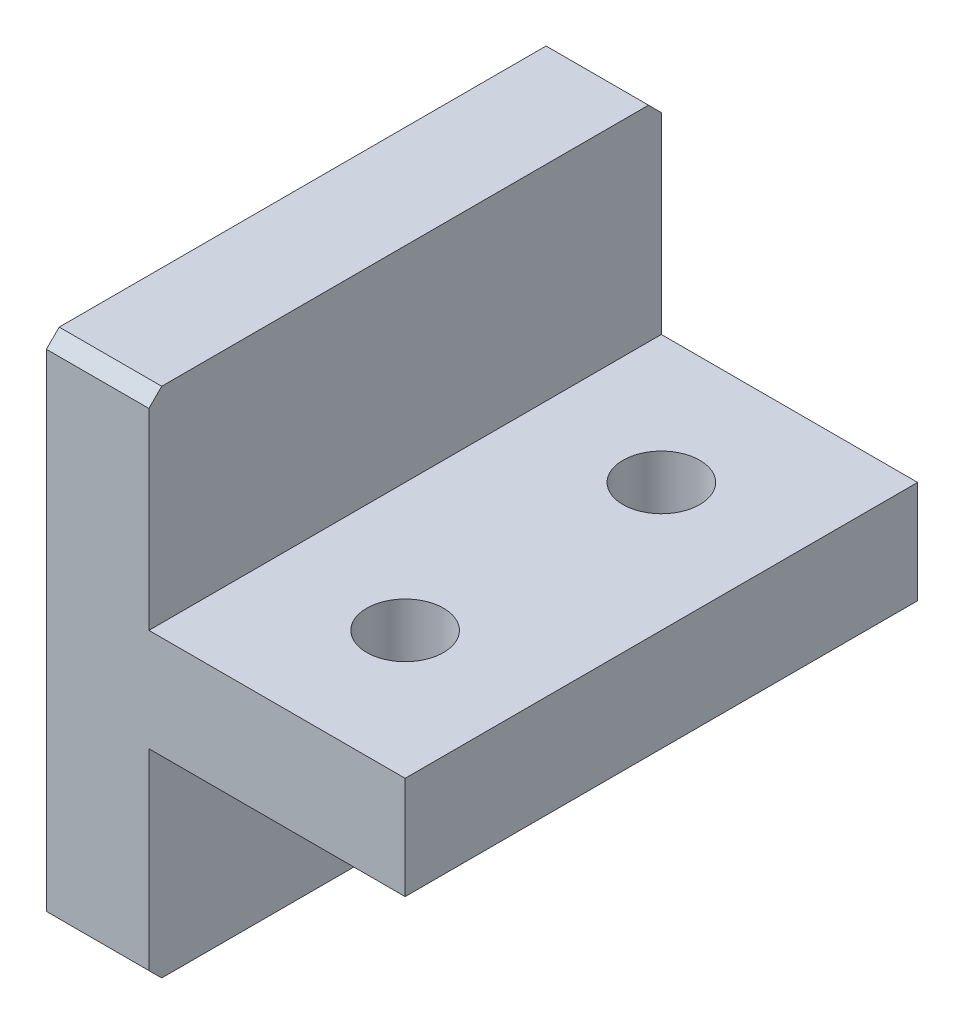
SolidWorks part; units mm, degrees
material "Q235-A"
ref_plane "Front Plane" through (0, 0, 0) normal (0, 0, 1) x (1, 0, 0)
ref_plane "Top Plane" through (0, 0, 0) normal (0, 1, 0) x (1, 0, 0)
ref_plane "Right Plane" through (0, 0, 0) normal (1, 0, 0) x (0, 0, -1)
sketch "Sketch1" plane through (0, 0, 0) normal (0, 1, 0) x (1, 0, 0)
  line L1 (0, 0) -> (8, 0)
  line L2 (0, 0) -> (0, -40)
  line L3 (0, -40) -> (8, -40)
  line L4 (8, 0) -> (8, -40)
  dimension "D1" = 8
  dimension "D2" = 40
extrude "Boss-Extrude1" add sketch "Sketch1" along normal blind 40
chamfer "Chamfer1" distance 1 angle 45 4 edges at (4, 40, 40) (4, 0, 40) (4, 40, 0) (4, 0, 0)
sketch "Sketch2" plane through (0, 0, 40) normal (0, 0, 1) x (1, 0, 0)
  line L0 (8, 39) -> (8, 1) construction
  line L1 (28, 24) -> (8, 24)
  line L2 (28, 24) -> (28, 16)
  line L3 (28, 16) -> (8, 16)
  line L4 (8, 24) -> (8, 16)
  line L6 (0, 1) -> (8, 1) construction
  point P10 (8, 20)
  dimension "D1" = 8
  dimension "D2" = 20
  dimension "D3" = 19
extrude "Boss-Extrude2" add sketch "Sketch2" against normal blind 40
sketch "Sketch4" plane through (0, 24, 0) normal (0, 1, 0) x (1, 0, 0)
  line L0 (8, -20) -> (18, -20) construction
  line L1 (8, 0) -> (8, -40) construction
  line L2 (18, -20) -> (18, -30) construction
  circle A0 centre (18, -30) radius 3
  circle A1 centre (18, -10) radius 3
extrude "Cut-Extrude1" cut sketch "Sketch4" against normal through all both and the other way through all
